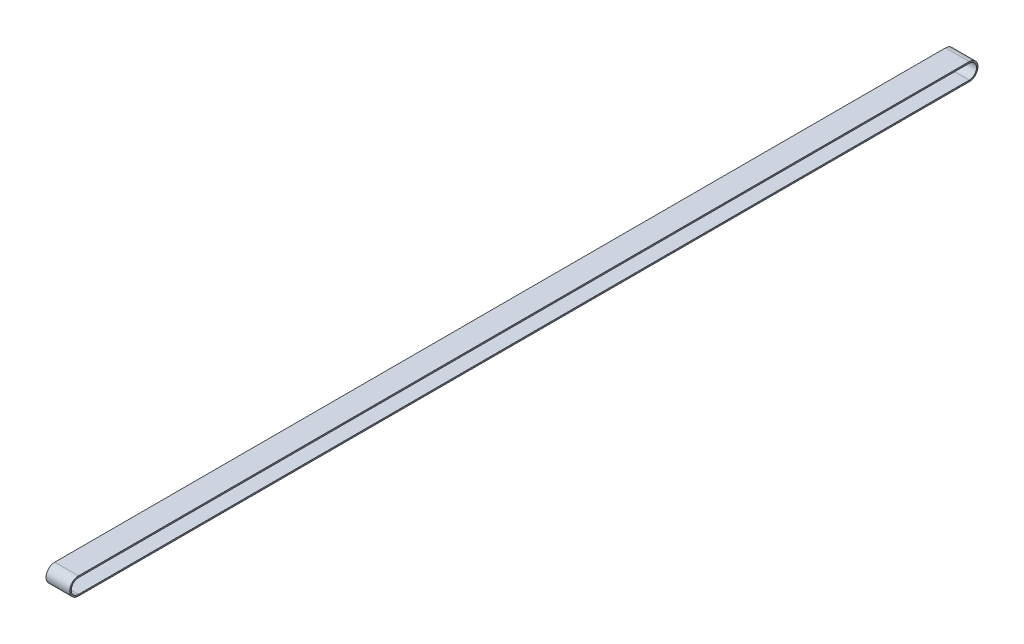
from build123d import *

# Parameters (mm, degrees)
EXTRUDE_1_DEPTH = 40
EXTRUDE_2_DEPTH = 40


with BuildPart() as part:
    # 草图1 → 拉伸-薄壁1 (new, symmetric)
    with BuildSketch(Plane(origin=(0, 0, 0), x_dir=(0, 0, -1), z_dir=(1, 0, 0))):
        with BuildLine():
            Line((3002.5, -29.575), (0, -29.575))
            ThreePointArc((0, -29.575), (-29.575, 0), (0, 29.575))
            Line((0, 29.575), (3002.5, 29.575))
            ThreePointArc((3002.5, 29.575), (3032.075, 0), (3002.5, -29.575))
        make_face()
        with BuildLine():
            Line((3002.5, -27.325), (0, -27.325))
            ThreePointArc((0, -27.325), (-27.325, 0), (0, 27.325))
            Line((0, 27.325), (3002.5, 27.325))
            ThreePointArc((3002.5, 27.325), (3029.825, 0), (3002.5, -27.325))
        make_face(mode=Mode.SUBTRACT)
    extrude(amount=EXTRUDE_1_DEPTH, both=True)


with BuildPart() as body_2:
    # 草图2 → 拉伸-薄壁2 (new, symmetric)
    with BuildSketch(Plane(origin=(0, 0, 0), x_dir=(0, 0, -1), z_dir=(1, 0, 0))):
        with BuildLine():
            Line((0, -27.325), (3002.5, -27.325))
            ThreePointArc((3002.5, -27.325), (3029.825, 0), (3002.5, 27.325))
            Line((3002.5, 27.325), (0, 27.325))
            ThreePointArc((0, 27.325), (-27.325, 0), (0, -27.325))
        make_face()
        with BuildLine():
            Line((0, -24.495), (3002.5, -24.495))
            ThreePointArc((3002.5, -24.495), (3026.995, 0), (3002.5, 24.495))
            Line((3002.5, 24.495), (0, 24.495))
            ThreePointArc((0, 24.495), (-24.495, 0), (0, -24.495))
        make_face(mode=Mode.SUBTRACT)
    extrude(amount=EXTRUDE_2_DEPTH, both=True)


solid = Compound([part.part, body_2.part])
